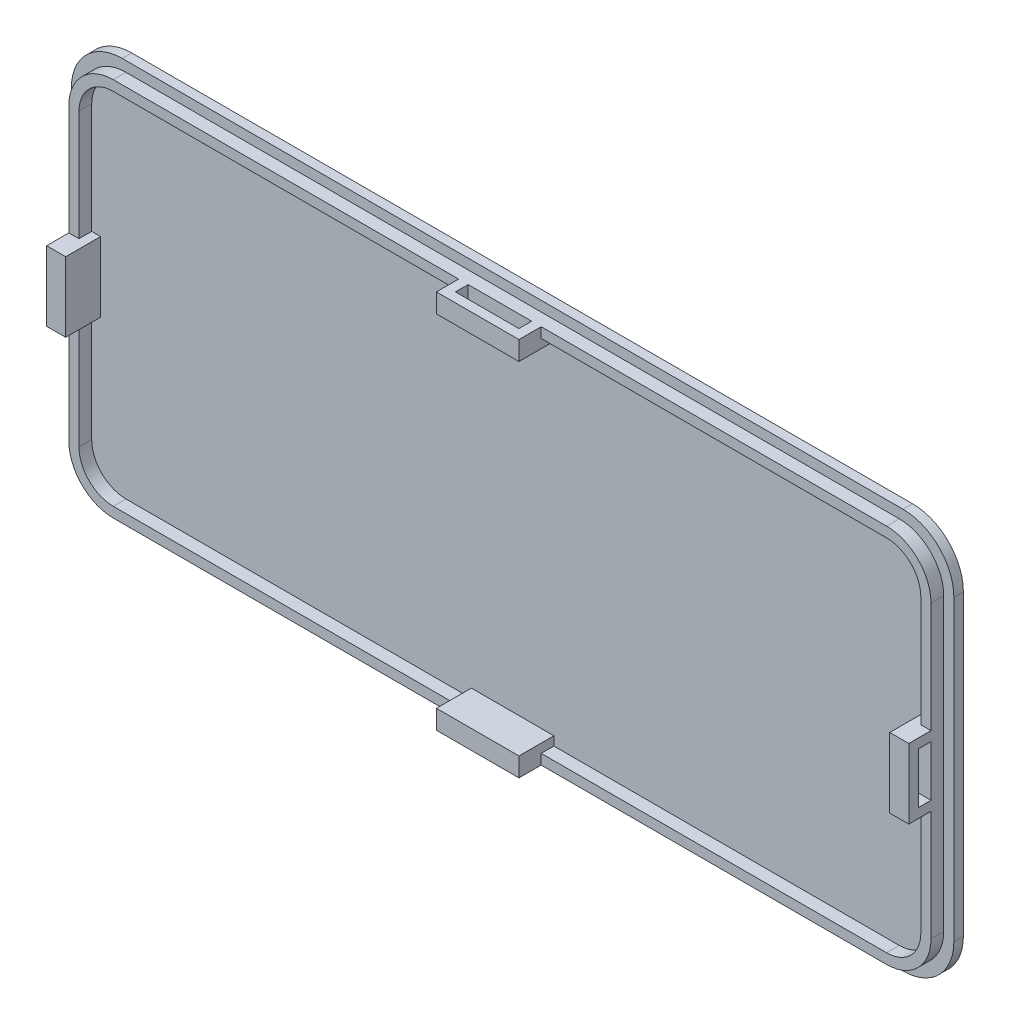
from build123d import *

# Parameters (mm, degrees)
BOSS_EXTRUDE1_DEPTH = 1.5
BOSS_EXTRUDE2_START = -1.5
SKETCH2_R           = 6
SKETCH2_R_2         = 5.1
BOSS_EXTRUDE2_DEPTH = 1
BOSS_EXTRUDE3_DEPTH = 2
SKETCH4_W           = 13
SKETCH4_H           = 3
SKETCH4_W_2         = 3
SKETCH4_H_2         = 11
BOSS_EXTRUDE4_DEPTH = 3.5
SKETCH5_W           = 10
SKETCH5_H           = 2
CUT_EXTRUDE1_DEPTH  = 2
SKETCH7_W           = 2
SKETCH7_H           = 19.411603012
CUT_EXTRUDE3_DEPTH  = 0.8
CUT_EXTRUDE4_START  = -1
SKETCH8_R           = 5.1
CUT_EXTRUDE4_DEPTH  = 1
SKETCH9_W           = 2
SKETCH9_H           = 8
CUT_EXTRUDE5_DEPTH  = 2


with BuildPart() as part:
    # Sketch1 → Boss-Extrude1 (new body)
    with BuildSketch(Plane.XY):
        with BuildLine():
            Line((-61.5, 31.5), (61.5, 31.5))
            ThreePointArc((61.5, 31.5), (67.156854249, 29.156854249), (69.5, 23.5))
            Line((69.5, 23.5), (69.5, -23.5))
            ThreePointArc((69.5, -23.5), (67.156854249, -29.156854249), (61.5, -31.5))
            Line((61.5, -31.5), (-61.5, -31.5))
            ThreePointArc((-61.5, -31.5), (-67.156854249, -29.156854249), (-69.5, -23.5))
            Line((-69.5, -23.5), (-69.5, 23.5))
            ThreePointArc((-69.5, 23.5), (-67.156854249, 29.156854249), (-61.5, 31.5))
        make_face()
    extrude(amount=BOSS_EXTRUDE1_DEPTH)

    # Sketch2 → Boss-Extrude2 (add)
    # profile 1 of 4: a face of its own
    with BuildSketch(Plane.XY.offset(1.5).offset(BOSS_EXTRUDE2_START)):
        with Locations((-58, 18)):
            Circle(SKETCH2_R)
        with Locations((-58, 18)):
            Circle(SKETCH2_R_2, mode=Mode.SUBTRACT)
    # profile 2 of 4: a face of its own
    with BuildSketch(Plane.XY.offset(1.5).offset(BOSS_EXTRUDE2_START)):
        with Locations((58, 18)):
            Circle(SKETCH2_R)
        with Locations((58, 18)):
            Circle(SKETCH2_R_2, mode=Mode.SUBTRACT)
    # profile 3 of 4: a face of its own
    with BuildSketch(Plane.XY.offset(1.5).offset(BOSS_EXTRUDE2_START)):
        with Locations((-58, -18)):
            Circle(SKETCH2_R)
        with Locations((-58, -18)):
            Circle(SKETCH2_R_2, mode=Mode.SUBTRACT)
    # profile 4 of 4: a face of its own
    with BuildSketch(Plane.XY.offset(1.5).offset(BOSS_EXTRUDE2_START)):
        with Locations((58, -18)):
            Circle(SKETCH2_R)
        with Locations((58, -18)):
            Circle(SKETCH2_R_2, mode=Mode.SUBTRACT)
    extrude(amount=-BOSS_EXTRUDE2_DEPTH)

    # Sketch3 → Boss-Extrude3 (add)
    with BuildSketch(Plane.XY.offset(1.5)):
        with BuildLine():
            Line((60.9, 29.9), (-60.9, 29.9))
            ThreePointArc((-60.9, 29.9), (-65.849747468, 27.849747468), (-67.9, 22.9))
            Line((-67.9, 22.9), (-67.9, -22.9))
            ThreePointArc((-67.9, -22.9), (-65.849747468, -27.849747468), (-60.9, -29.9))
            Line((-60.9, -29.9), (60.9, -29.9))
            ThreePointArc((60.9, -29.9), (65.849747468, -27.849747468), (67.9, -22.9))
            Line((67.9, -22.9), (67.9, 22.9))
            ThreePointArc((67.9, 22.9), (65.849747468, 27.849747468), (60.9, 29.9))
        make_face()
        with BuildLine():
            Line((60.9, 28.3), (-60.9, 28.3))
            ThreePointArc((-60.9, 28.3), (-64.718376618, 26.718376618), (-66.3, 22.9))
            Line((-66.3, 22.9), (-66.3, -22.9))
            ThreePointArc((-66.3, -22.9), (-64.718376618, -26.718376618), (-60.9, -28.3))
            Line((-60.9, -28.3), (60.9, -28.3))
            ThreePointArc((60.9, -28.3), (64.718376618, -26.718376618), (66.3, -22.9))
            Line((66.3, -22.9), (66.3, 22.9))
            ThreePointArc((66.3, 22.9), (64.718376618, 26.718376618), (60.9, 28.3))
        make_face(mode=Mode.SUBTRACT)
    extrude(amount=BOSS_EXTRUDE3_DEPTH)

    # Sketch4 → Boss-Extrude4 (add, symmetric)
    with BuildSketch(Plane.XY.offset(3.5)):
        with Locations((0, 28.4)):
            Rectangle(SKETCH4_W, SKETCH4_H)
        with Locations((0, -28.4)):
            Rectangle(SKETCH4_W, SKETCH4_H)
        with Locations((66.4, 0)):
            Rectangle(SKETCH4_W_2, SKETCH4_H_2)
        with Locations((-66.4, 0)):
            Rectangle(SKETCH4_W_2, SKETCH4_H_2)
    extrude(amount=BOSS_EXTRUDE4_DEPTH, both=True)

    # Sketch5 → Cut-Extrude1 (cut)
    with BuildSketch(Plane(origin=(0, 29.9, 0), x_dir=(1, 0, 0), z_dir=(0, 1, 0))):
        with Locations((0, -4.5)):
            Rectangle(SKETCH5_W, SKETCH5_H)
    cut_extrude1 = extrude(amount=-CUT_EXTRUDE1_DEPTH, mode=Mode.SUBTRACT)

    # Mirror1: Cut-Extrude1 across plane
    add(cut_extrude1.mirror(Plane.ZX), mode=Mode.SUBTRACT)

    # Sketch7 → Cut-Extrude3 (cut)
    with BuildSketch(Plane(origin=(0, -31.5, 0), x_dir=(-1, 0, 0), z_dir=(0, -1, 0))):
        Rectangle(SKETCH7_W, SKETCH7_H)
    extrude(amount=-CUT_EXTRUDE3_DEPTH, mode=Mode.SUBTRACT)

    # Sketch8 → Cut-Extrude4 (cut)
    with BuildSketch(Plane(origin=(0, 0, 0), x_dir=(-1, 0, 0), z_dir=(0, 0, -1)).offset(CUT_EXTRUDE4_START)):
        with Locations(Location((-58, 18, 0), (0, 0, 180))):
            Circle(SKETCH8_R)
        with Locations(Location((58, 18, 0), (0, 0, 180))):
            Circle(SKETCH8_R)
        with Locations(Location((58, -18, 0), (0, 0, 180))):
            Circle(SKETCH8_R)
        with Locations(Location((-58, -18, 0), (0, 0, 180))):
            Circle(SKETCH8_R)
    extrude(amount=CUT_EXTRUDE4_DEPTH, mode=Mode.SUBTRACT)

    # Sketch9 → Cut-Extrude5 (cut)
    with BuildSketch(Plane(origin=(67.9, 0, 0), x_dir=(0, 0, -1), z_dir=(1, 0, 0))):
        with Locations((-4.5, 0)):
            Rectangle(SKETCH9_W, SKETCH9_H)
    cut_extrude5 = extrude(amount=-CUT_EXTRUDE5_DEPTH, mode=Mode.SUBTRACT)

    # Mirror2: Cut-Extrude5 across plane
    add(cut_extrude5.mirror(Plane(origin=(0, 0, 0), x_dir=(0, 0, 1), z_dir=(1, 0, 0))), mode=Mode.SUBTRACT)


solid = part.part
